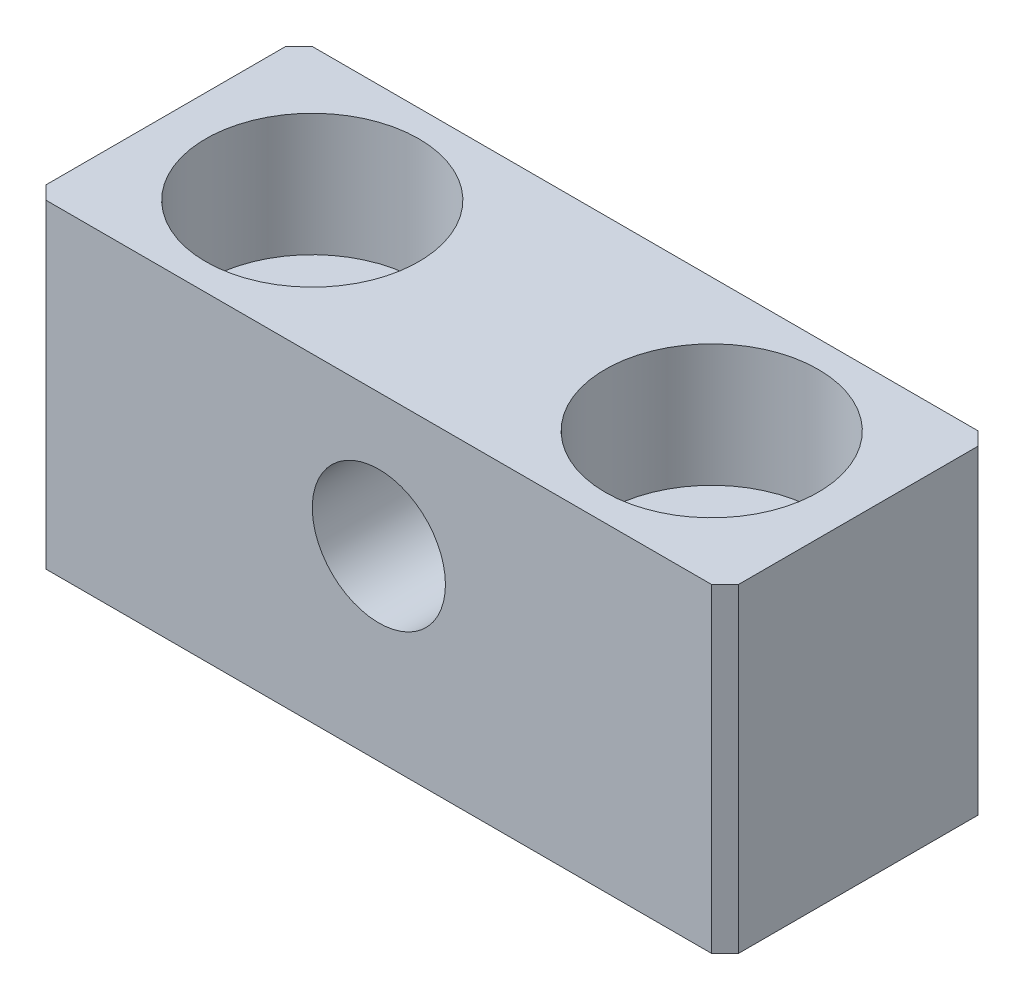
SolidWorks part; units mm, degrees
material "S45C"
ref_plane "前视基准面" through (0, 0, 0) normal (0, 0, 1) x (1, 0, 0)
ref_plane "上视基准面" through (0, 0, 0) normal (0, 1, 0) x (1, 0, 0)
ref_plane "右视基准面" through (0, 0, 0) normal (1, 0, 0) x (0, 0, -1)
sketch "草图1" plane through (0, 0, 0) normal (0, 0, 1) x (1, 0, 0)
  line L1 (-13, 6) -> (13, 6)
  line L2 (-13, 6) -> (-13, -6)
  line L3 (-13, -6) -> (13, -6)
  line L4 (13, 6) -> (13, -6)
  line L5 (-13, 6) -> (13, -6) construction
  line L6 (-13, -6) -> (13, 6) construction
  point P0 (0, 0)
  dimension "D1" = 26
  dimension "D2" = 12
extrude "凸台-拉伸1" add sketch "草图1" along normal mid plane 10
hole_wizard "打孔尺寸(%根据)内六角圆柱头螺钉的类型1" positions "草图3" profile "草图2" counterbore size "M4" standard "GB" end condition through all
sketch "草图3" plane through (0, 6, 0) normal (0, 1, 0) x (1, 0, 0)
  line L0 (0, 0) -> (0, 5) construction
  line L1 (13, 5) -> (-13, 5) construction
  point P0 (-7.5, 0)
  point P2 (7.5, 0)
  dimension "D1" = 15
sketch "草图2" plane through (-7.5, 6, 0) normal (1, 0, 0) x (0, 0, 1)
  line L0 (0, 0) -> (0, 12)
  line L1 (0, 12) -> (2.25, 12)
  line L3 (2.25, 12) -> (2.25, 4.6)
  line L4 (2.25, 4.6) -> (4, 4.6)
  line L5 (4, 4.6) -> (4, 0)
  line L7 (4, 0) -> (0, 0)
  line L11 (0, -6.35) -> (0, 107.95) construction
  dimension "通孔孔直径" = 4.5
  dimension "通孔孔深度" = 12
  dimension "柱形沉头孔直径" = 8
  dimension "柱形沉头孔深度" = 4.6
hole_wizard "M6 螺纹孔1" positions "草图5" profile "草图6" tap size "M6" standard "GB" end condition through all
sketch "草图5" plane through (0, 0, 5) normal (0, 0, 1) x (1, 0, 0)
  line L0 (-13, -6) -> (13, -6) construction
  point P0 (0, 1)
  dimension "D1" = 7
sketch "草图6" plane through (0, 1, 5) normal (1, 0, 0) x (0, -1, 0)
  line L0 (0, 0) -> (0, 10)
  line L1 (0, 10) -> (2.5, 10)
  line L2 (2.5, 10) -> (2.5, 0)
  line L5 (2.5, 0) -> (0, 0)
  line L11 (0, -6.35) -> (0, 107.95) construction
  dimension "通孔螺纹孔钻头直径" = 5
  dimension "通孔螺纹孔钻头深度" = 10
cosmetic thread "孔螺蚊线1" parameters "D2"=6
chamfer "倒角1" distance 0.5 angle 45 4 edges at (-13, 0, -5) (-13, 0, 5) (13, 0, -5) (13, 0, 5)
